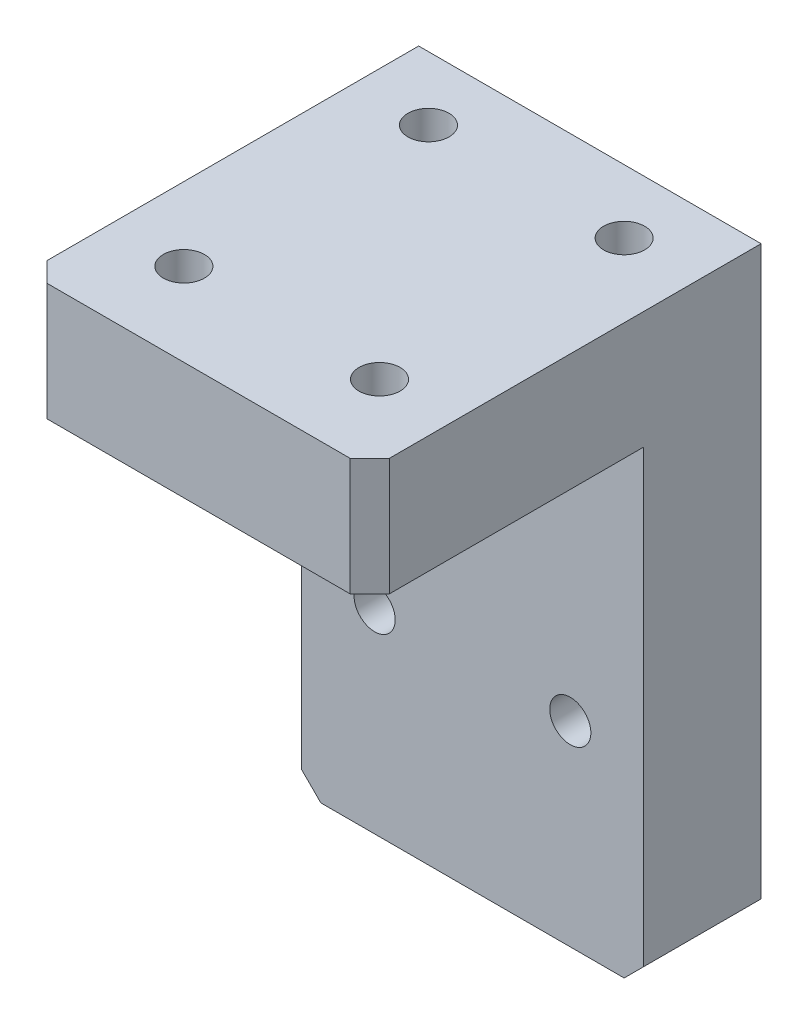
from build123d import *

# Parameters (mm, degrees)
SKETCH_1_W             = 35
SKETCH_1_H             = 60
EXTRUDE_1_DEPTH        = 12
CHAMFER_1_SIZE         = 2
SKETCH_4_W             = 28
SKETCH_4_H             = 12
EXTRUDE_2_DEPTH        = 35
HOLE_WIZARD_M5_1_D     = 4.2
CHAMFER_2_SIZE         = 2
HOLE_WIZARD_M5_2_D     = 4.2
HOLE_WIZARD_M5_2_DEPTH = 12.4
HOLE_WIZARD_M5_2_TIP   = 1.2618073


with BuildPart() as part:
    # 草图1 → 凸台-拉伸1 (new body)
    with BuildSketch(Plane.XY):
        Rectangle(SKETCH_1_W, SKETCH_1_H)
    extrude(amount=EXTRUDE_1_DEPTH)

    # 倒角1
    chamfer_1_edges = [part.edges().sort_by_distance(p)[0] for p in [
        (-17.5, -30, 6),
        (17.5, -30, 6),
    ]]
    chamfer(chamfer_1_edges, length=CHAMFER_1_SIZE)

    # 草图4 → 凸台-拉伸2 (add)
    with BuildSketch(Plane.ZY.offset(17.5)):
        with Locations((26, 24)):
            Rectangle(SKETCH_4_W, SKETCH_4_H)
    extrude(amount=-EXTRUDE_2_DEPTH)

    # M5 螺纹孔1 (through all)
    with Locations(Plane(origin=(0, 0, 0), x_dir=(-1, 0, 0), z_dir=(0, 0, -1))):
        with Locations((-10, -10), (10, -10)):
            Hole(HOLE_WIZARD_M5_1_D / 2)

    # 倒角2
    chamfer_2_edges = [part.edges().sort_by_distance(p)[0] for p in [
        (-17.5, 24, 40),
        (17.5, 24, 40),
    ]]
    chamfer(chamfer_2_edges, length=CHAMFER_2_SIZE)

    # M5 螺纹孔2
    with Locations(Plane(origin=(0, 30, 0), x_dir=(1, 0, 0), z_dir=(0, 1, 0))):
        with Locations((-10, -6.5), (10, -6.5), (-10, -31.5), (10, -31.5)):
            Hole(HOLE_WIZARD_M5_2_D / 2, depth=HOLE_WIZARD_M5_2_DEPTH)
            with Locations((0, 0, -(HOLE_WIZARD_M5_2_DEPTH + HOLE_WIZARD_M5_2_TIP / 2))):  # 118° drill point
                Cone(0, HOLE_WIZARD_M5_2_D / 2, HOLE_WIZARD_M5_2_TIP, mode=Mode.SUBTRACT)


solid = part.part
